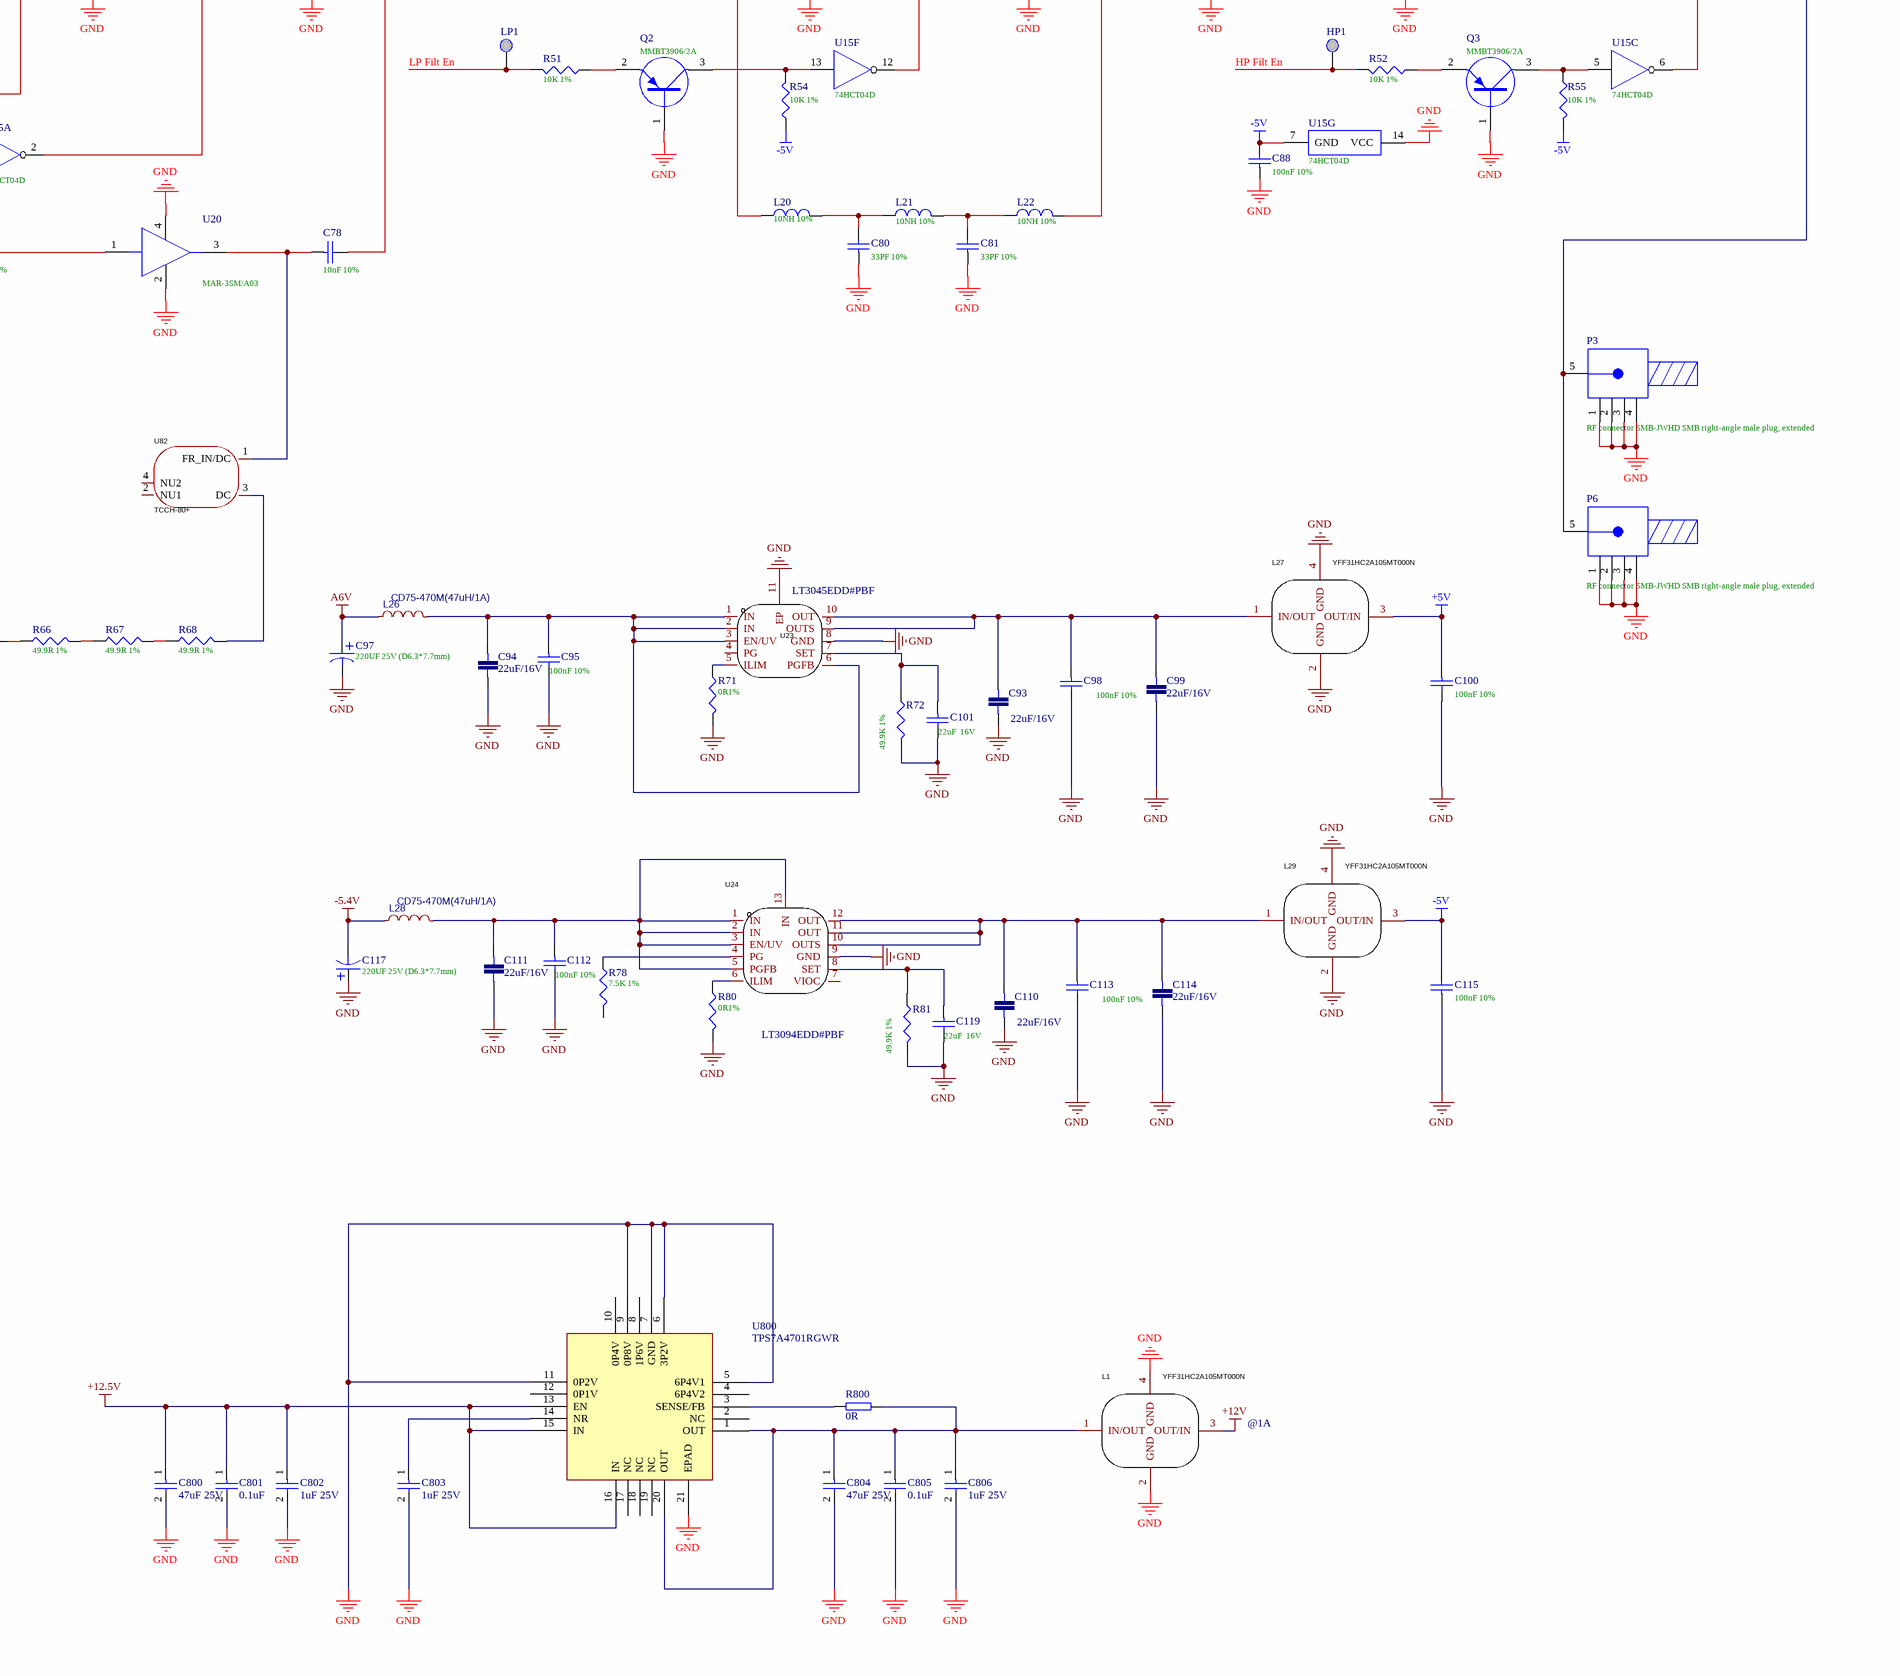
[diagram p0: PCBE109560-6.SchDoc, bottom right]
# Altium schematic sheet PCBE109560-6.SchDoc (part 2 of 2)

## Parts
1  (no value)  [DIP-1]
+1  (no value)  [DIP-1]
+2  (no value)  [DIP-1]
C4  20PF 10%  [0805C]
C5  330PF 10%  [1812C]
C6  22PF 10%  [1812C-2]
C7  22uF/16V  [0805]
C8  22uF/16V  [0805]
C9  100nF 10%  [0603]
C10  220UF 25V (D6.3*7.7mm)  [CAP-SMD_BD6.3-L6.6-W6.6-FD]
C11  100nF 10%  [0603]
C12  22uF/16V  [0805]
C13  100nF 10%  [0805R]
C14  22uF  16V  [0805]
C15  100nF 10%  [0805R]
C16  47PF 10%  [1812C-2]
C17  100PF 10%  [1812C-2]
C18  20PF 10%  [0805R]
C20  100nF 10%  [0805R]
C21  100nF 10%  [0805R]
C31  100nF 10%  [0805R]
C32  100nF 10%  [0805R]
C34  100nF 10%  [0805R]
C35  100nF 10%  [0805R]
C36  100nF 10%  [0805R]
C37  100nF 10%  [0805R]
C39  100nF 10%  [0805R]
C40  100nF 10%  [0805R]
C41  100nF 10%  [0805R]
C42  100nF 10%  [0805R]
C43  100nF 10%  [0805R]
C44  100nF 10%  [0805R]
C45  100nF 10%  [0805R]
C46  100nF 10%  [0805R]
C47  100nF 10%  [0805R]
C48  100nF 10%  [0805R]
C49  22uF 25V  [CAP-SMD_L6.0-W3.2-R-RD]
C50  100nF 10%  [0805R]
C51  100nF 10%  [0805R]
C52  100nF 10%  [0805R]
C53  3.3NF 10%  [0805R]
C54  100nF 10%  [0805R]
C55  330PF 10%  [0805R]
C56  330PF 10%  [0805R]
C57  100nF 10%  [0805R]
C58  33PF 10%  [0805R]
C59  33PF 10%  [0805R]
C60  100nF 10%  [0805R]
C61  100nF 10%  [0805R]
C62  100nF 10%  [0805R]
C63  100nF 10%  [0805R]
C64  100nF 10%  [0805R]
C65  33PF 10%  [0805R]
C66  33PF 10%  [0805R]
C67  100nF 10%  [0805R]
C68  39PF 10%  [0805R]
C69  100nF 10%  [0805R]
C70  25V 1UF Type A  [0805C-2]
C71  25V 1UF Type A  [0805C-2]
C72  100nF 10%  [0805R]
C73  25V 1UF Type A  [0805C-2]
C74  100nF 10%  [0805R]
C75  100nF 10%  [0805R]
C76  10nF 10%  [0805R]
C77  10nF 10%  [0805R]
C78  10nF 10%  [0805R]
C79  100nF 10%  [0603C]
C80  33PF 10%  [0805R]
C81  33PF 10%  [0805R]
C82  100nF 10%  [0805R]
C83  100nF 10%  [0805R]
C84  100nF 10%  [0805R]
C85  100nF 10%  [0805R]
C86  25V 1UF Type A  [0805C-2]
C87  3pF( ±0.1pF)  [0805R]
C88  100nF 10%  [0805R]
C89  100nF 10%  [0805R]
C90  100nF 10%  [0805R]
C93  22uF/16V  [0805]
C94  22uF/16V  [0805]
C95  100nF 10%  [0603]
C96  100nF 10%  [0805R]
C97  220UF 25V (D6.3*7.7mm)  [CAP-SMD_BD6.3-L6.6-W6.6-FD]
C98  100nF 10%  [0603]
C99  22uF/16V  [0805]
C100  100nF 10%  [0805R]
C101  22uF  16V  [0805]
C102  100nF 10%  [0805R]
C103  100nF 10%  [0805R]
C104  100nF 10%  [0805R]
C105  100nF 10%  [0805R]
C106  100nF 10%  [0805R]
C107  100nF 10%  [0805R]
C109  100nF 10%  [0805R]
C110  22uF/16V  [0805]
C111  22uF/16V  [0805]
C112  100nF 10%  [0603]
C113  100nF 10%  [0603]
C114  22uF/16V  [0805]
C115  100nF 10%  [0805R]
C116  100nF 10%  [0805R]
C117  220UF 25V (D6.3*7.7mm)  [CAP-SMD_BD6.3-L6.6-W6.6-FD]
C118  100nF 10%  [0805R]
C119  22uF  16V  [0805]
C122  100nF 10%  [0805R]
C123  100nF 10%  [0805R]
C124  100nF 10%  [0805R]
C125  100nF 10%  [0805R]
C128  100nF 10%  [0805R]
C129  100nF 10%  [0805R]
C130  100nF 10%  [0805R]
C800  47uF 25V  [1206]
C801  0.1uF  [0402]
C802  1uF 25V  [0402]
C803  1uF 25V  [0402]
C804  47uF 25V  [1206]
C805  0.1uF  [0402]
C806  1uF 25V  [0402]
Clk1  (no value)  [DIP-1]
D1  BAV99/A7  [SOT-23]
D2  GF1M-E3/67A/GM  [1808D]
D3  GF1M-E3/67A/GM  [1808D]
D4  GF1M-E3/67A/GM  [1808D]
D5  GF1M-E3/67A/GM  [1808D]
D8  BAV99/A7  [SOT-23-2]
D9  BAV99/A7  [SOT-23-2]
D10  BAV99/A7  [SOT-23-2]
D11  BAV99/A7  [SOT-23-2]
D12  BAV99/A7  [SOT-23-2]
Data1  (no value)  [DIP-1]
HP1  (no value)  [DIP-1]
J1  RF connector  [DIP-P]
J2  RF connector  [DIP-P]
L1  YFF31HC2A105MT000N  [FILTER-SMD_4P-L3.2-W1.6-L_YFF31HC]
L2  15UH 5%  [1005R]
L3  BLM21PG221SN1D(220Ω@100MHz)  [0805R]
L4  YFF31HC2A105MT000N  [FILTER-SMD_4P-L3.2-W1.6-L_YFF31HC]
L5  6.8UH 10%  [0805R]
L8  YFF31HC2A105MT000N  [FILTER-SMD_4P-L3.2-W1.6-L_YFF31HC]
L10  10NH 10%  [0805R]
L11  10NH 10%  [0805R]
L12  10NH 10%  [0805R]
L13  YFF31HC2A105MT000N  [FILTER-SMD_4P-L3.2-W1.6-L_YFF31HC]
L15  4.7UH 5%  [1005L]
L16  1UH 5%  [0805R]
L17  BLM21PG221SN1D(220Ω@100MHz)  [0805R]
L18  BLM21PG221SN1D(220Ω@100MHz  [0805R]
L19  BLM21PG221SN1D(220Ω@100MHz  [0805R]
L20  10NH 10%  [0805R]
L21  10NH 10%  [0805R]
L22  10NH 10%  [0805R]
L23  YFF31HC2A105MT000N  [FILTER-SMD_4P-L3.2-W1.6-L_YFF31HC]
L24  YFF31HC2A105MT000N  [FILTER-SMD_4P-L3.2-W1.6-L_YFF31HC]
L25  BLM21PG221SN1D(220Ω@100MHz  [0805R]
L26  CD75-470M(47uH/1A)  [IND-SMD_L7.8-W7.0-A]
L27  YFF31HC2A105MT000N  [FILTER-SMD_4P-L3.2-W1.6-L_YFF31HC]
L28  CD75-470M(47uH/1A)  [IND-SMD_L7.8-W7.0-A]
L29  YFF31HC2A105MT000N  [FILTER-SMD_4P-L3.2-W1.6-L_YFF31HC]
L31  BLM21PG221SN1D(220Ω@100MHz  [0805R]
L32  BLM21PG221SN1D(220Ω@100MHz  [0805R]
L808  NFM15PC104R1A3D  [FILTER-SMD_0402-3P-L1.0-W0.5-T]
L809  NFM15PC104R1A3D  [FILTER-SMD_0402-3P-L1.0-W0.5-T]
L810  NFM15PC104R1A3D  [FILTER-SMD_0402-3P-L1.0-W0.5-T]
L811  NFM15PC104R1A3D  [FILTER-SMD_0402-3P-L1.0-W0.5-T]
L812  NFM15PC104R1A3D  [FILTER-SMD_0402-3P-L1.0-W0.5-T]
L813  NFM15PC104R1A3D  [FILTER-SMD_0402-3P-L1.0-W0.5-T]
LP1  (no value)  [DIP-1]
P1  Header 20X2  [N0.8mm/40Pin-Plug]
P2  Header 4X2  [N0.8mm/8Pin-SOCKET]
P3  RF connector SMB-JWHD SMB right-angle male plug, extended  [DIP-P-2]
P4  Header 20X2  [N0.8mm/40Pin-Plug]
P5  Header 20X2  [N0.8mm/40Pin-Plug]
P6  RF connector SMB-JWHD SMB right-angle male plug, extended  [DIP-P-2]
Q1  MJD31C  [SOT-252-2]
Q2  MMBT3906/2A  [SOT-23]
Q3  MMBT3906/2A  [SOT-23]
Q4  MMBT3906/2A  [SOT-23]
R6  2K 5%  [0603R]
R7  NC  [AXIAL-0.51]
R8  3.9K 5% 1/2W  [AXIAL-0.51]
R9  3.9K 5% 1/2W  [AXIAL-0.51]
R10  3.9K 5% 1/2W  [AXIAL-0.51]
R11  3.9K 5% 1/2W  [AXIAL-0.51]
R13  0R1%  [0603]
R14  49.9K 1%  [0603]
R15  4.99K 1%  [0805R]
R16  2K 1%  [0805R]
R17  49.9R 1% 1/4W  [AXIAL-0.4]
R20  100R 1% 1/4W  [AXIAL-0.4]
R23  100R 1% 1/4W  [AXIAL-0.4]
R27  4.87K 1%  [0805R]
R28  4.87K 1%  [0805R]
R29  4.87K 1%  [0805R]
R30  4.87K 1%  [0805R]
R31  4.87K 1%  [0805R]
R32  10K 1%  [0805R]
R33  100K 1%  [0805R]
R34  100K 1%  [0805R]
R35  49.9R 1%  [0805R]
R36  49.9R 1%  [0805R]
R37  49.9R 1%  [0805R]
R38  49.9R 1%  [0805R]
R39  49.9R 1%  [0805R]
R40  49.9R 1% 1/4W  [R-SMD_L3.5-W1.5]
R41  10K 1%  [0805R]
R42  4.87K 1%  [0805R]
R43  4.87K 1%  [0805R]
R44  4.87K 1%  [0805R]
R45  4.87K 1%  [0805R]
R46  169R 1%  [0805R]
R47  169R 1%  [0805R]
R48  169R 1%  [0805R]
R49  49.9R 1%  [0805R]
R50  49.9R 1%  [0805R]
R51  10K 1%  [0805R]
R52  10K 1%  [0805R]
R53  10K 1%  [0805R]
R54  10K 1%  [0805R]
R55  10K 1%  [0805R]
R56  10K 1%  [0805R]
R57  10K 1%  [0805R]
R58  49.9R 1%  [0805R]
R59  4.99K 1%  [0805R]
R60  49.9R 1%  [R-SMD_L3.5-W1.5]
R61  30R 1%  [R-SMD_L3.5-W1.5]
R62  169R 1%  [0805R]
R63  169R 1%  [0805R]
R64  169R 1%  [0805R]
R65  49.9R 1%  [0805R]
R66  49.9R 1%  [0805R]
R67  49.9R 1%  [0805R]
R68  49.9R 1%  [0805R]
R69  120R 1%  [R-SMD_L3.5-W1.5]
R70  169R 1%  [0805R]
R71  0R1%  [0603]
R72  49.9K 1%  [0603]
R73  169R 1%  [0805R]
R74  NC  [0805R]
R75  169R 1%  [0805R]
R77  169R 1%  [0805R]
R78  7.5K 1%  [0603]
R80  0R1%  [0603]
R81  49.9K 1%  [0603]
R82  100K 1%  [0805R]
R83  10K 1%  [0805R]
R84  169R 1%  [0805R]
R800  0R  [0402]
RE1  AGQ210A4HZ  [RELAY-SMD_PANASONIC_AGQ2X0AXX]
RE2  AGQ210A4HZ  [RELAY-SMD_PANASONIC_AGQ2X0AXX]
RE3  AGQ210A4HZ  [RELAY-SMD_PANASONIC_AGQ2X0AXX]
RE4  AGQ210A4HZ  [RELAY-SMD_PANASONIC_AGQ2X0AXX]
RE5  AGQ210A4HZ  [RELAY-SMD_PANASONIC_AGQ2X0AXX]
Strobe1  (no value)  [DIP-1]
U4  LT3045EDD#PBF  [DFN-10_L3.0-W3.0-P0.50-BL-EP]
U6  74HCT123D  [SOIC-16_L9.9-W3.9-P1.27-LS6.0-BL]
U8  MAX504CSD+T  [SO-14]
U9  SW-239  [SO-8]
U11  SW-239  [SO-8]
U12  SW-239  [SO-8]
U13  SW-239  [SO-8]
U14  SW-239  [SO-8]
U15  74HCT04D  [SO-14]  (parts A,B,C,D,E,F,G of 7)
U16  AT-250(MAAV-007941)  [SO-8]
U17  MAR-3SM/A03  [LCC4]
U18  MAR-6SM/A06  [LCC4]
U19  MAR-6SM/A06  [LCC4]
U20  MAR-3SM/A03  [LCC4]
U21  MAX4106ESA+T  [SO-8]
U22  MIC4420CM  [SO-8]
U23  LT3045EDD#PBF  [DFN-10_L3.0-W3.0-P0.50-BL-EP]
U24  LT3094EDD#PBF  [WDFN-12_L3.0-W3.0-P0.45-BL-EP]
U25  AT65-0263  [SO-16]
U80  TCCH-80+  [IND-SMD_4P-L3.8-W3.8]
U81  TCCH-80+  [IND-SMD_4P-L3.8-W3.8]
U82  TCCH-80+  [IND-SMD_4P-L3.8-W3.8]
U83  TCCH-80+  [IND-SMD_4P-L3.8-W3.8]
U100  SW-239  [SO-8]
U800  TPS7A4701RGWR  [QFN-20]

## Nets
+5V: C100.1 L27.3(OUT/IN) L808.3(OUTPUT) L811.3(OUTPUT) L812.3(OUTPUT) U8.3(~{CLR})
+12.5V: +2.1 C106.1 C800.1 C801.1 C802.1 P5.31 P5.32 P5.33 P5.34 P5.35 P5.36 P5.37 P5.38 P5.39 P5.40 U800.13(EN) U800.15(IN) U800.16(IN)
+12V: C122.1 C123.1 C124.2 C125.2 L1.3(OUT/IN) L8.1(IN/OUT) L13.1(IN/OUT) U22.1(VS) U22.8(VS)
-5.4V: +1.1 C107.1 C117.2 L28.2 P5.1 P5.2 P5.3 P5.4 P5.5 P5.6 P5.7 P5.8 P5.9 P5.10
-5V: C88.2 C115.2 L29.3(OUT/IN) L809.1(INPUT) L810.3(OUTPUT) L813.3(OUTPUT) R54.1 R55.2 R57.1 U15.7(GND)
A6V: 1.1 C10.1 C97.1 C103.2 L3.1 L26.2 P5.17 P5.18 P5.19 P5.20 P5.21 P5.22 P5.23 P5.24
GND: C5.1 C6.2 C7.1 C8.1 C9.2 C10.2 C11.2 C12.1 C13.2 C14.2 C15.1 C18.2 C20.1 C21.1 C31.1 C32.1 C34.1 C35.1 C36.2 C37.2 C39.2 C40.2 C42.2 C43.1 C44.2 C45.2 C46.2 C47.1 C48.1 C49.2 C50.2 C57.2 C60.2 C61.1 C62.1 C63.1 C64.1 C65.2 C66.1 C70.1 C71.1 C72.2 C73.1 C74.1 C75.1 C80.1 C81.1 C83.2 C84.2 C85.1 C86.2 C88.1 C89.2 C90.2 C93.1 C94.1 C95.2 C96.2 C97.2 C98.2 C99.1 C100.2 C101.2 C102.2 C103.1 C104.2 C105.1 C106.2 C107.2 C109.2 C110.1 C111.1 C112.2 C113.2 C114.1 C115.1 C117.1 C118.2 C119.2 C122.2 C123.2 C124.1 C125.1 C128.1 C129.1 C130.2 C800.2 C801.2 C802.2 C803.2 C804.2 C805.2 C806.2 D1.3 D2.2(K) D11.2 D12.1 J1.1 J1.2 J1.3 J1.4 J2.1 J2.2 J2.3 J2.4 L1.2(GND) L1.4(GND) L2.2 L4.2(GND) L4.4(GND) L8.2(GND) L8.4(GND) L13.2(GND) L13.4(GND) L15.2 L16.1 L23.2(GND) L23.4(GND) L24.2(GND) L24.4(GND) L27.2(GND) L27.4(GND) L29.2(GND) L29.4(GND) L808.2(GND) L809.2(GND) L810.2(GND) L811.2(GND) L812.2(GND) L813.2(GND) P1.5 P1.6 P1.11 P1.12 P1.17 P1.18 P1.20 P1.23 P1.24 P1.29 P1.30 P1.35 P1.36 P2.1 P2.3 P2.5 P2.7 P3.1 P3.2 P3.3 P3.4 P4.5 P4.6 P4.11 P4.12 P4.17 P4.18 P4.23 P4.24 P4.29 P4.30 P4.35 P4.36 P5.11 P5.12 P5.13 P5.14 P5.15 P5.16 P5.25 P5.26 P5.27 P5.28 P5.29 P5.30 P6.1 P6.2 P6.3 P6.4 Q1.2(E) Q2.1(B) Q3.1(B) Q4.1(B) R13.2 R14.2 R20.2 R32.2 R53.1 R59.1 R61.1 R71.2 R72.2 R74.1 R80.2 R81.2 R82.1 R83.1 RE1.3 RE3.6 RE4.2 U4.8(GND) U4.11(EP) U6.6(2CEXT) U6.8(GND) U6.10(2B) U6.14(1CEXT) U8.7(DGND) U8.8(AGND) U9.2(GND) U9.7(GND) U9.8(GND) U11.2(GND) U11.7(GND) U11.8(GND) U12.2(GND) U12.7(GND) U12.8(GND) U13.2(GND) U13.7(GND) U13.8(GND) U14.2(GND) U14.7(GND) U14.8(GND) U15.14(VCC) U16.2(GND) U16.3(GND) U16.5(GND) U16.6(GND) U16.7(GND) U17.2(GND) U17.4(GND) U18.2(GND) U18.4(GND) U19.2(GND) U19.4(GND) U20.2(GND) U20.4(GND) U22.4(GND) U22.5(GND) U23.8(GND) U23.11(EP) U24.9(GND) U25.2(GND) U25.3(GND) U25.4(GND) U25.5(GND) U25.6(GND) U25.7(GND) U25.16(GND) U100.2(GND) U100.7(GND) U100.8(GND) U800.5(6P4V1) U800.6(3P2V) U800.7(GND) U800.9(0P8V) U800.11(0P2V) U800.21(EPAD)
VCC: C13.1 C15.2 L4.3(OUT/IN) R15.1 R16.2 U6.2(1B) U6.3(1~{R}D) U6.16(VCC)
AK2: C21.2 P1.33 RE1.1
AK3: C20.2 P1.38 RE1.8
AK4: C37.1 P1.37 RE2.1
AK5: C36.1 P1.40 RE2.8
AK6: C31.2 P1.34 RE3.8
AK7: C32.2 P1.32 RE3.1
AK8: C34.2 C40.1 P1.28 RE4.8 RE5.8
AK9: C35.2 C39.1 P1.26 RE4.1 RE5.1
Attn1: P4.34 R70.2
Attn2: P4.32 R73.2
Attn4: P4.28 R75.2
Attn8: P4.26 R77.2
Attn16: P4.22 R84.2
DAC Clk: Clk1.1 P4.14 U8.4(SCLK)
DAC Data: Data1.1 P4.16 U8.2(DIN)
DAC Strobe: P4.10 Strobe1.1 U8.5(~{CS})
DATA_T: P1.39 R15.2 U6.1(1~{A})
HP Filt En: HP1.1 P4.4 R52.2
HT: L5.1 P2.2 P2.4 P2.6 P2.8
IN2: P4.8 R56.1 U22.2(IN)
LP Filt En: LP1.1 P4.2 R51.2
NetC4_1: C4.1 D1.2 L2.1 Q1.1(B) R6.1
NetC4_2: C4.2 R6.2 U6.13(1Q)
NetC5_2: C5.2 L5.2 R7.2
NetC6_1: C6.1 C16.2 C17.2 Q1.3(C) R11.1
NetC7_2: C7.2 C11.1 C12.2 L4.1(IN/OUT) U4.9(OUTS) U4.10(OUT)
NetC8_2: C8.2 C9.1 L3.2 U4.1(IN) U4.2(IN) U4.3(EN/UV) U4.6(PGFB)
NetC14_1: C14.1 R14.1 U4.7(SET)
NetC16_1: C16.1 D5.1(A) D8.2 D9.2 RE2.6
NetC17_1: C17.1 RE2.7
NetC18_1: C18.1 R16.1 U6.15(1REXT/CEXT)
NetC41_1: C41.1 U14.1(RFCOM)
NetC41_2: C41.2 P3.5 P6.5 R32.1
NetC42_1: C42.1 R27.1 U9.5(B)
NetC43_2: C43.2 R28.2 U100.4(A)
NetC44_1: C44.1 R29.1 U11.4(A)
NetC45_1: C45.1 R30.1 U12.5(B)
NetC46_1: C46.1 R31.1 U13.5(B) U14.4(A)
NetC47_2: C47.2 R35.1 U16.4(A)
NetC48_2: C48.2 L8.3(OUT/IN) R36.1
NetC49_1: C49.1 C50.1 U8.1(BIPOFF) U8.9(REFIN) U8.10(REFOUT)
NetC51_1: C51.1 U17.1(RF_IN)
NetC51_2: C51.2 U16.8(RF2)
NetC52_1: C52.1 L10.2
NetC52_2: C52.2 U17.3(RF_OUT) U81.1(FR_IN/DC)
NetC53_1: C53.1 C54.1 L15.1
NetC53_2: C53.2 U12.1(RFCOM)
NetC54_2: C54.2 U13.1(RFCOM)
NetC55_1: C55.1 U13.3(RF1)
NetC55_2: C55.2 C56.1 L16.2
NetC56_2: C56.2 U14.6(RF2)
NetC57_1: C57.1 R41.1 U13.4(A) U14.5(B)
NetC58_1: C58.1 C65.1
NetC58_2: C58.2 L10.1 L11.1
NetC59_1: C59.1 L11.2 L12.1
NetC59_2: C59.2 C66.2
NetC60_1: C60.1 R42.1 U9.4(A)
NetC61_2: C61.2 R43.2 U100.5(B)
NetC62_2: C62.2 R44.1 U11.5(B)
NetC63_2: C63.2 R45.1 U12.4(A)
NetC64_2: C64.2 L13.3(OUT/IN) R46.2
NetC67_1: C67.1 U18.1(RF_IN)
NetC67_2: C67.2 U25.1(RF)
NetC68_1: C68.1 C69.2 R49.2 R50.2
NetC68_2: C68.2 R49.1 R50.1 U18.3(RF_OUT) U80.1(FR_IN/DC)
NetC69_1: C69.1 R53.2 U16.1(RF1)
NetC70_2: C70.2 C74.2 L18.1 L19.2
NetC71_2: C71.2 C75.2 L19.1 U21.4(VEE)
NetC72_1: C72.1 C73.2 L17.2 L18.2
NetC76_1: C76.1 U9.3(RF1)
NetC76_2: C76.2 U19.1(RF_IN)
NetC77_1: C77.1 U19.3(RF_OUT) U83.1(FR_IN/DC)
NetC77_2: C77.2 U20.1(RF_IN)
NetC78_1: C78.1 U20.3(RF_OUT) U82.1(FR_IN/DC)
NetC78_2: C78.2 U100.6(RF2)
NetC79_1: C79.1 D10.3 R40.2
NetC79_2: C79.2 R58.2 R59.2
NetC80_2: C80.2 L20.2 L21.2
NetC81_2: C81.2 L21.1 L22.1
NetC82_1: C82.1 R60.2
NetC82_2: C82.2 C116.1 R74.2 R82.2
NetC83_1: C83.1 C86.1 L25.2 U21.7(VCC)
NetC84_1: C84.1 L23.3(OUT/IN) R62.2
NetC85_2: C85.2 L24.3(OUT/IN) R65.1
NetC87_1: C87.1 R60.1 R69.1 U21.6(OUT)
NetC87_2: C87.2 R61.2 R69.2 U21.2(IN-)
NetC89_1: C89.1 L813.1(INPUT) U8.11(VSS)
NetC90_1: C90.1 L32.2 L811.1(INPUT)
NetC93_2: C93.2 C98.1 C99.2 L27.1(IN/OUT) U23.9(OUTS) U23.10(OUT)
NetC94_2: C94.2 C95.1 L26.1 U23.1(IN) U23.2(IN) U23.3(EN/UV) U23.6(PGFB)
NetC96_1: C96.1 R70.1 U25.15(C1)
NetC101_1: C101.1 R72.1 U23.7(SET)
NetC102_1: C102.1 R73.1 U25.14(C2)
NetC104_1: C104.1 L812.1(INPUT) U8.13(VDD)
NetC105_2: C105.2 L31.1 L810.1(INPUT)
NetC109_1: C109.1 R75.1 U25.13(C4)
NetC110_2: C110.2 C113.1 C114.2 L29.1(IN/OUT) U24.10(OUTS) U24.11(OUT) U24.12(OUT)
NetC111_2: C111.2 C112.1 L28.1 U24.1(IN) U24.2(IN) U24.3(EN/UV) U24.5(PGFB) U24.13(IN)
NetC116_2: C116.2 R83.2 U25.8(RF)
NetC118_1: C118.1 R77.1 U25.12(C8)
NetC119_1: C119.1 R81.1 U24.8(SET)
NetC128_2: C128.2 L31.2 U25.11(VEE)
NetC129_2: C129.2 L32.1 U25.10(VCC)
NetC130_1: C130.1 R84.1 U25.9(C16)
NetC803_1: C803.1 U800.14(NR)
NetC804_1: C804.1 C805.1 C806.1 L1.1(IN/OUT) R800.1 U800.1(OUT) U800.20(OUT)
NetD2_1: D2.1(A) D3.2(K)
NetD3_1: D3.1(A) D4.2(K)
NetD4_1: D4.1(A) D5.2(K)
NetD8_1: D8.1 D9.1 J1.5 R17.1 R20.1 R23.1 RE4.4
NetD10_1: D10.1 D12.2
NetD10_2: D10.2 D11.1
NetJ2_5: J2.5 RE5.4
NetL12_2: L12.2 U9.1(RFCOM)
NetL17_1: L17.1 L809.3(OUTPUT)
NetL20_1: L20.1 U11.6(RF2)
NetL22_2: L22.2 U12.3(RF1)
NetL23_1: L23.1(IN/OUT) L24.1(IN/OUT) U22.6(OUT) U22.7(OUT)
NetL25_1: L25.1 L808.1(INPUT)
NetQ2_2: Q2.2(E) R51.1
NetQ2_3: Q2.3(C) R54.2 U15.13(6A)
NetQ3_2: Q3.2(E) R52.1
NetQ3_3: Q3.3(C) R55.1 U15.5(3A)
NetQ4_2: Q4.2(E) R56.2
NetQ4_3: Q4.3(C) R57.2 U15.1(1A)
NetR7_1: R7.1 R8.1
NetR8_2: R8.2 R9.2
NetR9_1: R9.1 R10.1
NetR10_2: R10.2 R11.2
NetR13_1: R13.1 U4.5(ILIM)
NetR17_2: R17.2 RE1.2
NetR23_2: R23.2 RE3.7
NetR27_2: R27.2 R28.1 U15.4(2Y)
NetR29_2: R29.2 R30.2 U15.10(5Y)
NetR31_2: R31.2 U15.8(4Y)
NetR33_1: R33.1 R34.1 U8.14(RFB)
NetR33_2: R33.2 R34.2 R35.2 U8.12(VOUT)
NetR36_2: R36.2 R37.1
NetR37_2: R37.2 R38.2
NetR38_1: R38.1 R39.1
NetR39_2: R39.2 U81.3(DC)
NetR40_1: R40.1 RE5.3
NetR41_2: R41.2 U15.6(3Y) U15.9(4A)
NetR42_2: R42.2 R43.1 U15.2(1Y) U15.3(2A)
NetR44_2: R44.2 R45.2 U15.11(5A) U15.12(6Y)
NetR46_1: R46.1 R47.2
NetR47_1: R47.1 R48.1
NetR48_2: R48.2 U80.3(DC)
NetR58_1: R58.1 U21.3(IN+)
NetR62_1: R62.1 R63.1
NetR63_2: R63.2 R64.2
NetR64_1: R64.1 U83.3(DC)
NetR65_2: R65.2 R66.2
NetR66_1: R66.1 R67.1
NetR67_2: R67.2 R68.1
NetR68_2: R68.2 U82.3(DC)
NetR71_1: R71.1 U23.5(ILIM)
NetR78_1: R78.1 U24.4(PG)
NetR80_1: R80.1 U24.6(ILIM)
NetR800_2: R800.2 U800.3(SENSE/FB)
NetRE4_3: RE4.3 RE5.2
NetU9_6: U9.6(RF2) U100.3(RF1)
NetU11_1: U11.1(RFCOM) U100.1(RFCOM)
NetU11_3: U11.3(RF1) U12.6(RF2)
NetU13_6: U13.6(RF2) U14.3(RF1)

Not connected (* = marked no-connect by the designer): D1 1*; D8 3; D9 3; D11 3; D12 3; P1 1 2 3 4 7 8 9 10 13 14 15 16 19 21 22 25 27 31; P4 1 3 7 9 13 15 19 20 21 25 27 31 33 37 38 39 40; R78 2; RE1 4 5 6 7; RE2 2 3 4 5; RE3 2 3 4 5; RE4 5 6 7; RE5 5 6 7; U4 4(PG); U6 4(1~{Q}) 5(2Q) 7(2REXT/CEXT) 9(2~{A}) 11(2~{R}D) 12(2~{Q}); U8 6(DOUT); U22 3(NC); U23 4(PG); U24 7(VIOC); U80 2(NU1) 4(NU2); U81 2(NU1) 4(NU2); U82 2(NU1) 4(NU2); U83 2(NU1) 4(NU2); U800 2(NC) 4(6P4V2) 8(1P6V) 10(0P4V) 12(0P1V) 17(NC) 18(NC) 19(NC)

## Notes on the sheet
- (near P1) Transmit interface
- 500V high-voltage interface
- Receive interface
- @1A

## Library data of the parts
1 +1 +2 Clk1 Data1 HP1 LP1 Strobe1 = TP
C4-C6 C9 C11 C13-C18 C20 C21 C31 C32 C34-C37 C39-C48 C50-C69 C72-C85 C87-C90 C95 C96 C98 C100-C107 C109 C112 C113 C115 C116 C118 C119 C122-C125 C128-C130 C800-C806 = CAP: Capacitor
C7 C8 C12 C93 C94 C99 C110 C111 C114 = C1206
C10 C97 C117 = CAPACITOR_1: Capacitor
C49 = TAJC226K025RNJ: Manufacturer: Kyocera AVX; Add into BOM: yes; Tolerance: ±10%; Equivalent Series Resistance(ESR): 1.4Ω@100kHz; Symbol: TAJC226K025RNJ; Device: TAJC226K025RNJ; LCSC Part Name: 22uF ±10% 25V; Supplier Part: C7214; Manufacturer Part: TAJC226K025RNJ; Supplier Footprint: CASE-C-6032; JLCPCB Part Class: Extended Part; Datasheet: https://atta.szlcsc.com/upload/public/pdf/source/20160107/1457707750344.pdf; Supplier: LCSC; Convert to PCB: yes; Value: 22uF; Rated Voltage: 25V; Operating Temperature: -55℃~+125℃
C70 C71 C86 = CAPACITOR POL: Capacitor
D1 D8-D12 = BAV99
D2-D5 = DIODE
J1 J2 = SMA-KWE: BOM_Supplier: *; BOM_Supplier Part: *; BOM_Manufacturer: *; BOM_Manufacturer Part: *; BOM_JLCPCB Part Class: *; spicePre: *; spiceSymbolName: *; Contributor: *
L1 L4 L8 L13 L23 L24 L27 L29 = YFF31HC2A105MT000N: Manufacturer: TDK; Add into BOM: yes; Nominal Capacitance: 1uF; CapacitanceTolerance: ±20%; DC Rated Voltage: 100V; Rated Current: 6A; DC Resistance: 5mΩ; Name: YFF31HC2A105MT000N; Symbol: YFF31HC2A105MT000N; Device: YFF31HC2A105MT000N; LCSC Part Name: 1uF(105) ±20% 100V; Supplier Part: C113216; Manufacturer Part: YFF31HC2A105MT000N; Supplier Footprint: SMD-4P,1.6x3.2mm; JLCPCB Part Class: Extended Part; Datasheet: https://atta.szlcsc.com/upload/public/pdf/source/20180326/C113216_F6F81E50B9805DA3D7C436129903DEBD.pdf; Supplier: LCSC; Convert to PCB: yes; Operating Temperature: -55℃~+125℃
L2 L3 L5 L10-L12 L15-L22 L25 L31 L32 = INDUCTOR
L26 L28 = 4.7uH/5a: BOM_Manufacturer: COILMX; BOM_Manufacturer Part: MS0630-4R7M; nameAlias: Inductance; Contributor: LCSC; BOM_Supplier: LCSC; BOM_Supplier Part: C380177; spicePre: L; spiceSymbolName: MS0630-4R7M
L808-L813 = NFM15PC104R1A3D: Manufacturer: muRata(村田); Add into BOM: yes; Nominal Capacitance: 100nF; CapacitanceTolerance: ±20%; DC Rated Voltage: 10V; Rated Current: 2A; DC Resistance: 30mΩ; Symbol: NFM15PC104R1A3D; Device: NFM15PC104R1A3D; LCSC Part Name: 0.1uF ±20% 10V; Supplier Part: C2650905; Manufacturer Part: NFM15PC104R1A3D; Supplier Footprint: 0402; JLCPCB Part Class: Extended Part; Datasheet: https://atta.szlcsc.com/upload/public/pdf/source/20210611/05FD8D968916F804F398094FB2B4AAFE.pdf; Supplier: LCSC; Convert to PCB: yes; Operating Temperature: -55℃~+105℃; Comment_1: NFM15PC104R1A3D
P1 P4 P5 = Header 20X2: Header, 20-Pin, Dual row; LatestRevisionDate: 17-Jul-2002; LatestRevisionNote: Re-released for DXP Platform.; Publisher: Altium Limited
P2 = Header 4X2: Header, 4-Pin, Dual row; LatestRevisionDate: 17-Jul-2002; LatestRevisionNote: Re-released for DXP Platform.; Publisher: Altium Limited
P3 P6 = JA1
Q1 = NPN: NPN Transistor
Q2-Q4 = PNP: PNP Transistor
R6-R11 R13-R17 R20 R23 R27-R75 R77 R78 R80-R84 = RES1
R800 = RES
RE1-RE5 = AGQ210A4HZ: Manufacturer: PANASONIC(松下); Add into BOM: yes; Coil Voltage: 4.5V; Contact Form: Two changeover sets: 2C (DPDT changeover); Maximum Switching Voltage: 125V@AC; 110V@DC; Coil Type: Single coil; Maximum Switching Current: 2A; Operate Time: 4ms; Symbol: AGQ210A4HZ; Device: AGQ210A4HZ; LCSC Part Name: AGQ210A4HZ; Supplier Part: C2153577; Manufacturer Part: AGQ210A4HZ; Supplier Footprint: SMD,7.2x10.6mm; JLCPCB Part Class: Extended Part; Datasheet: https://atta.szlcsc.com/upload/public/pdf/source/20210727/C2858037_82AE1FE69E1888D41D6E9B5D42950540.pdf; Supplier: LCSC; Convert to PCB: yes; Pin Number: -; Contact Rating: -; Contact Material: AgPd + gold plating; Coil Rated Power: -; Coil Resistance: -; Release Time: 4ms; Contact Resistance: -; Operating Temperature: -40℃~+85℃; Comment_1: AGQ210A4HZ
U4 U23 = LT3045EDD#PBF: Symbol: LT3045EDD#PBF_C666574; Add into BOM: yes; Maximum Input Voltage: 20V; Output Voltage: 0V~15V; MAX Output Current: 500mA; Dropout Voltage: 450mV@(500mA); standby current: 20uA; Number of Outputs: 1; Device: LT3045EDD#PBF; LCSC Part Name: LT3045EDD#PBF; Supplier Part: C666574; Manufacturer Part: LT3045EDD#PBF; Supplier Footprint: DFN-10-EP(3x3); JLCPCB Part Class: Extended Part; Datasheet: https://atta.szlcsc.com/upload/public/pdf/source/20200416/C514420_E440C492D6C74EAE6AB301243586F696.pdf; Supplier: LCSC; Convert to PCB: yes
U15 = 74HC04
U16 = AT-250
U17 U20 = MAR-3SM
U18 U19 = MAR-6SM
U21 = MAX4107ESA: Manufacturer: *; Manufacturer Part: *; Supplier Part: *; Supplier: *; link: *; spicePre: *; spiceSymbolName: *; Package Display: *; Contributor: *
U24 = LT3094EDD#PBF: Add into BOM: yes; Symbol: LT3094EDD#PBF; Device: LT3094EDD#PBF; LCSC Part Name: LT3094EDD#PBF; Supplier Part: C670492; Manufacturer Part: LT3094EDD#PBF; Supplier Footprint: WDFN-12-EP(3x3); JLCPCB Part Class: Extended Part; Datasheet: https://atta.szlcsc.com/upload/public/pdf/source/20200318/C498217_A5485280C797CF3891C55BEBE66C21D4.pdf; Supplier: LCSC; Convert to PCB: yes; Output Type: -
U80-U83 = TCCH-80+: Manufacturer: Mini-Circuits; Add into BOM: yes; Value: 4uH; Rated Current: 200mA; DC Resistance (DCR): 100mΩ; Symbol: TCCH-80+; Device: TCCH-80+; LCSC Part Name: 4uH; Supplier Part: C3223029; Manufacturer Part: TCCH-80+; Supplier Footprint: SMD-4P,3.8x3.8mm; JLCPCB Part Class: Extended Part; Datasheet: https://atta.szlcsc.com/upload/public/pdf/source/20240402/75EC49D4FFFA61CBEC009CC2CCA83C83.pdf; Supplier: LCSC; Convert to PCB: yes; Tolerance: -; Saturation Current (Isat): -; Type: -; Ratings: -
U800 = TPS7A4701RGWR(QFN20): Name: *; Symbol: *; Device: *; LCSC Part Name: *; Supplier Part: *; Manufacturer: *; Manufacturer Part: *; Supplier Footprint: *; JLCPCB Part Class: *; Datasheet: *; Supplier: *; Add into BOM: *; Convert to PCB: *; Output Type: *; Output Polarity: *; Number of Outputs: *